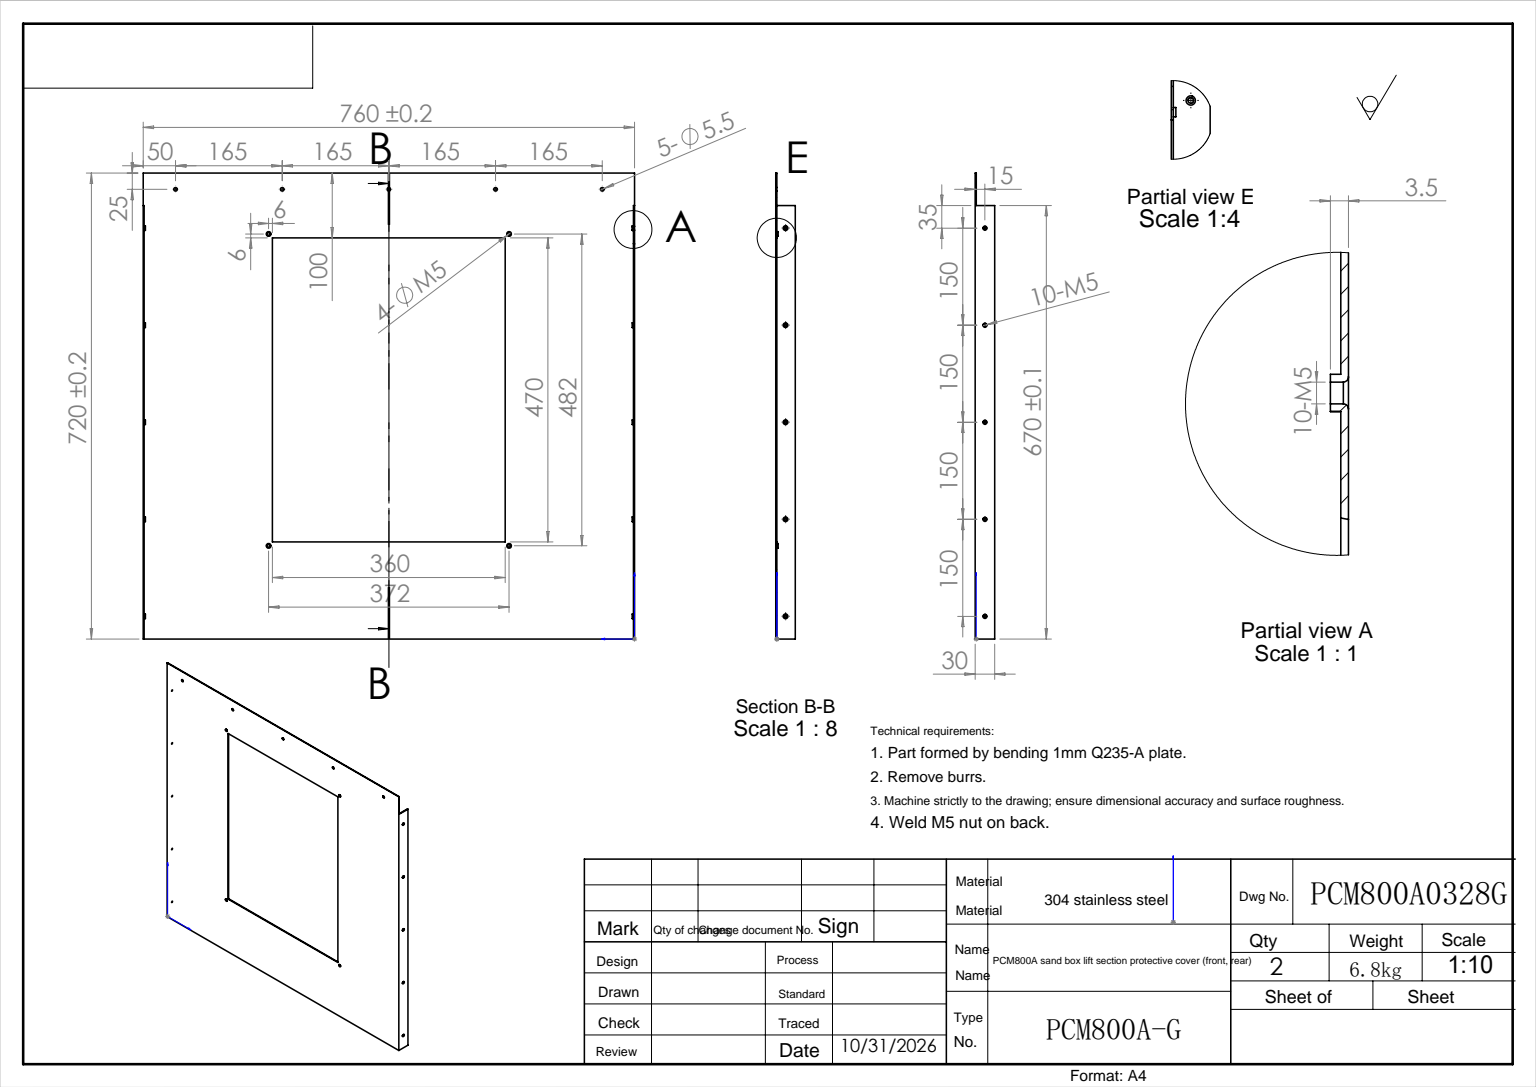
from build123d import *

# Parameters (mm, degrees)
SKETCH_1_W          = 760
SKETCH_1_H          = 720
EXTRUDE_1_DEPTH     = 1.5
SKETCH_2_W          = 1.5
SKETCH_2_H          = 670
EXTRUDE_2_DEPTH     = 28.5
SKETCH_3_R          = 2.75
CUT_EXTRUDE_1_DEPTH = 30
SKETCH_5_R          = 3.6
EXTRUDE_3_DEPTH     = 2
EXTRUDE_START       = 2
SKETCH_6_R          = 3.6
EXTRUDE_4_DEPTH     = 2
HOLE_WIZARD_M5_1_D  = 4.2
FILLET_2_R          = 1
SKETCH_9_W          = 360
SKETCH_9_H          = 470
CUT_EXTRUDE_2_DEPTH = 10
SKETCH_10_R         = 3.6
EXTRUDE_5_DEPTH     = 2
SKETCH_11_R         = 2.1
CUT_EXTRUDE_3_DEPTH = 112
FILLET_3_R          = 1


with BuildPart() as part:
    # 草图1 → 凸台-拉伸1 (new body)
    with BuildSketch(Plane.XY):
        with Locations((380, 360)):
            Rectangle(SKETCH_1_W, SKETCH_1_H)
    extrude(amount=EXTRUDE_1_DEPTH)

    # 草图2 → 凸台-拉伸2 (add)
    with BuildSketch(Plane(origin=(0, 0, 0), x_dir=(-1, 0, 0), z_dir=(0, 0, -1))):
        with Locations((-759.25, 335)):
            Rectangle(SKETCH_2_W, SKETCH_2_H)
        with Locations((-0.75, 335)):
            Rectangle(SKETCH_2_W, SKETCH_2_H)
    extrude(amount=EXTRUDE_2_DEPTH)

    # 草图3 → 切除-拉伸1 (cut)
    with BuildSketch(Plane(origin=(0, 0, 0), x_dir=(-1, 0, 0), z_dir=(0, 0, -1))):
        with Locations((-710, 695)):
            Circle(SKETCH_3_R)
        with Locations((-545, 695)):
            Circle(SKETCH_3_R)
        with Locations((-380, 695)):
            Circle(SKETCH_3_R)
        with Locations((-215, 695)):
            Circle(SKETCH_3_R)
        with Locations((-50, 695)):
            Circle(SKETCH_3_R)
    extrude(amount=-CUT_EXTRUDE_1_DEPTH, mode=Mode.SUBTRACT)

    # 草图5 → 凸台-拉伸3 (add)
    with BuildSketch(Plane(origin=(1.5, 0, 0), x_dir=(0, 0, -1), z_dir=(1, 0, 0))):
        with Locations(Location((13.5, 635, 0), (0, 0, 180))):
            Circle(SKETCH_5_R)
        with Locations(Location((13.5, 485, 0), (0, 0, 180))):
            Circle(SKETCH_5_R)
        with Locations(Location((13.5, 335, 0), (0, 0, 180))):
            Circle(SKETCH_5_R)
        with Locations(Location((13.5, 185, 0), (0, 0, 180))):
            Circle(SKETCH_5_R)
        with Locations(Location((13.5, 35, 0), (0, 0, 180))):
            Circle(SKETCH_5_R)
    extrude(amount=EXTRUDE_3_DEPTH)

    # 草图6 → 凸台-拉伸4 (add)
    with BuildSketch(Plane.ZY.offset(-758.5).offset(EXTRUDE_START)):
        with Locations((-13.5, 635)):
            Circle(SKETCH_6_R)
        with Locations((-13.5, 485)):
            Circle(SKETCH_6_R)
        with Locations((-13.5, 335)):
            Circle(SKETCH_6_R)
        with Locations((-13.5, 185)):
            Circle(SKETCH_6_R)
        with Locations((-13.5, 35)):
            Circle(SKETCH_6_R)
    extrude(amount=-EXTRUDE_4_DEPTH)

    # M5 螺纹孔1 (through all)
    with Locations(Plane.ZY):
        with Locations((-13.5, 635), (-13.5, 485), (-13.5, 335), (-13.5, 185), (-13.5, 35)):
            Hole(HOLE_WIZARD_M5_1_D / 2)

    # 圆角2
    fillet_2_edges = [part.edges().sort_by_distance(p)[0] for p in [
        (760, 35, -11.4),
        (0, 35, -11.4),
        (760, 185, -11.4),
        (0, 185, -11.4),
        (760, 335, -11.4),
        (0, 335, -11.4),
        (760, 485, -11.4),
        (0, 485, -11.4),
        (760, 635, -11.4),
        (0, 635, -11.4),
    ]]
    fillet(fillet_2_edges, radius=FILLET_2_R)

    # 草图9 → 切除-拉伸2 (cut)
    with BuildSketch(Plane.XY.offset(1.5)):
        with Locations((380, 385)):
            Rectangle(SKETCH_9_W, SKETCH_9_H)
    extrude(amount=-CUT_EXTRUDE_2_DEPTH, mode=Mode.SUBTRACT)

    # 草图10 → 凸台-拉伸5 (add)
    with BuildSketch(Plane(origin=(0, 0, 0), x_dir=(-1, 0, 0), z_dir=(0, 0, -1))):
        with Locations((-566, 626)):
            Circle(SKETCH_10_R)
        with Locations((-194, 626)):
            Circle(SKETCH_10_R)
        with Locations((-194, 144)):
            Circle(SKETCH_10_R)
        with Locations((-566, 144)):
            Circle(SKETCH_10_R)
    extrude(amount=EXTRUDE_5_DEPTH)

    # 草图11 → 切除-拉伸3 (cut)
    with BuildSketch(Plane(origin=(0, 0, -2), x_dir=(-1, 0, 0), z_dir=(0, 0, -1))):
        with Locations((-566, 626)):
            Circle(SKETCH_11_R)
        with Locations((-194, 626)):
            Circle(SKETCH_11_R)
        with Locations((-194, 144)):
            Circle(SKETCH_11_R)
        with Locations((-566, 144)):
            Circle(SKETCH_11_R)
    extrude(amount=-CUT_EXTRUDE_3_DEPTH, mode=Mode.SUBTRACT)

    # 圆角3
    fillet_3_edges = [part.edges().sort_by_distance(p)[0] for p in [
        (568.1, 626, 1.5),
        (196.1, 626, 1.5),
        (196.1, 144, 1.5),
        (568.1, 144, 1.5),
    ]]
    fillet(fillet_3_edges, radius=FILLET_3_R)


solid = part.part
